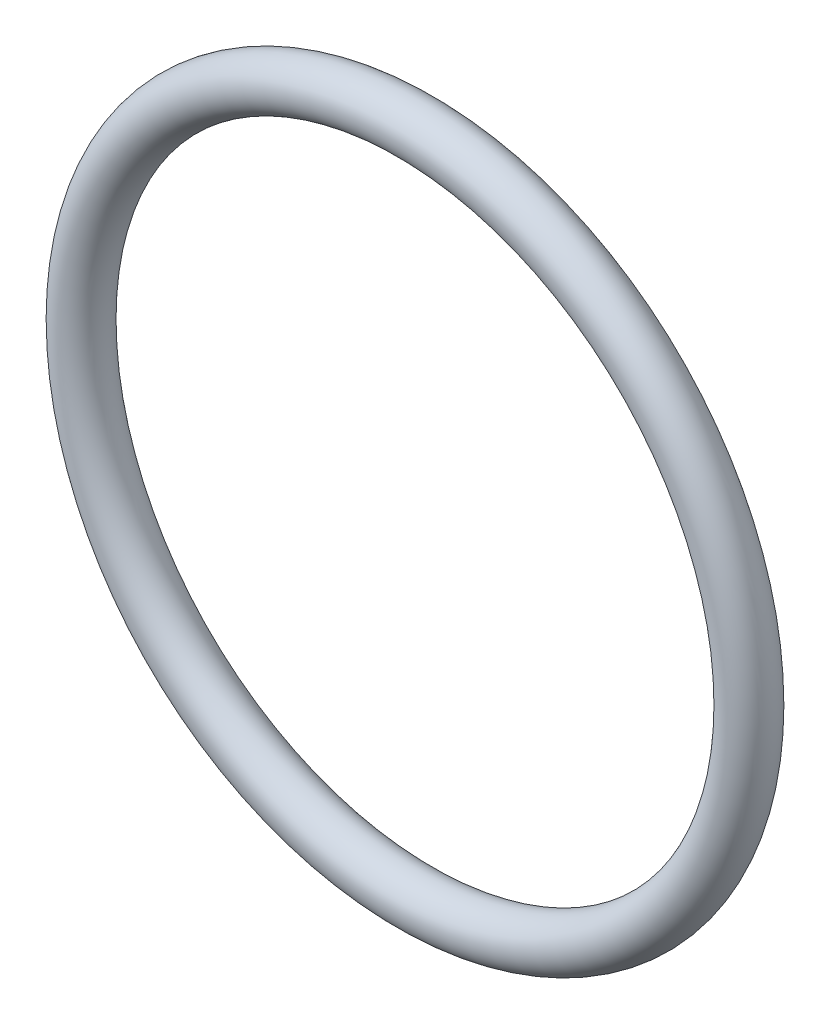
from build123d import *

# Parameters (mm, degrees)
SKETCH1_R = 1


with BuildPart() as part:
    # Sketch1 → Revolve1 (revolve)
    with BuildSketch(Plane(origin=(0, 0, 0), x_dir=(1, 0, 0), z_dir=(0, 1, 0))):
        with Locations((-13.5, 0)):
            Circle(SKETCH1_R)
    revolve(axis=Axis((0, 0, 0), (0, 0, 1)))


solid = part.part
